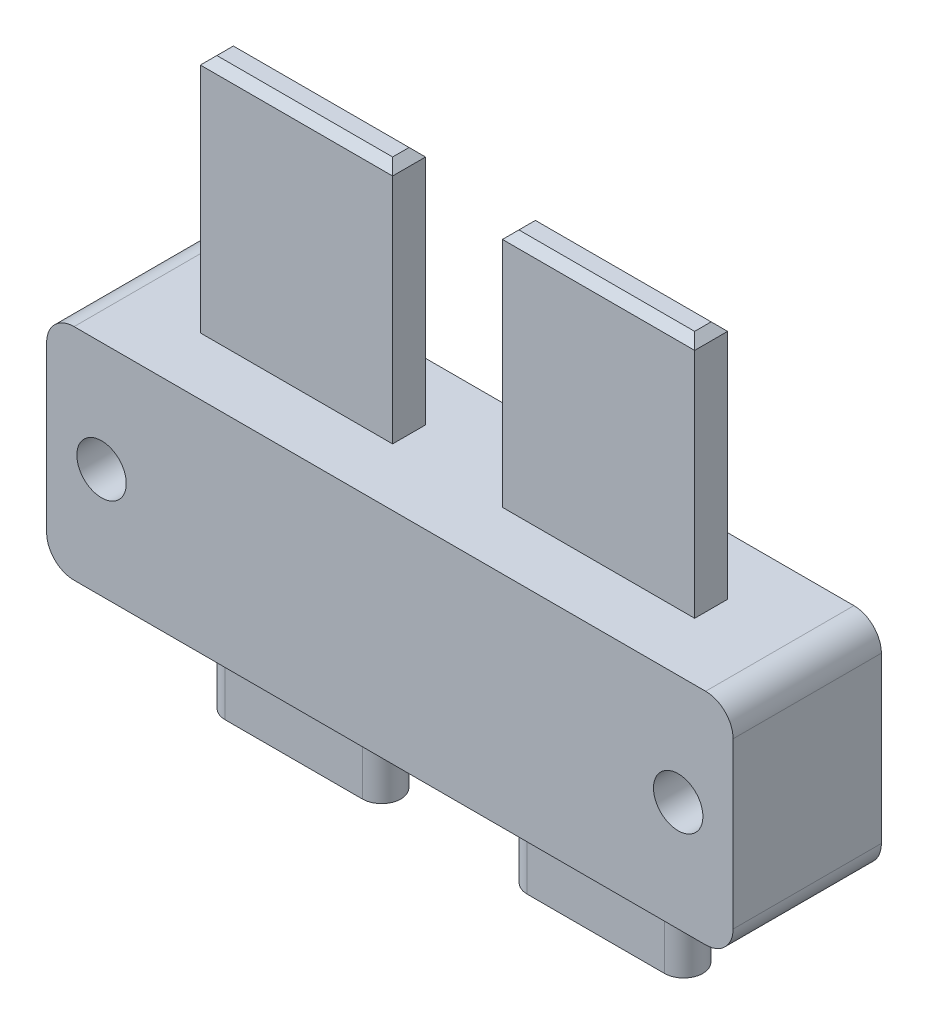
SolidWorks part; units mm, degrees
ref_plane "前视基准面" through (0, 0, 0) normal (0, 0, 1) x (1, 0, 0)
ref_plane "上视基准面" through (0, 0, 0) normal (0, 1, 0) x (1, 0, 0)
ref_plane "右视基准面" through (0, 0, 0) normal (1, 0, 0) x (0, 0, -1)
other "Configuration Table"
sketch "草图1" plane through (0, 0, 0) normal (0, 0, 1) x (1, 0, 0)
  line L0 (0, 0) -> (24.1432, 0) construction
  line L1 (-12.5, 4) -> (12.5, 4)
  line L2 (-12.5, 4) -> (-12.5, -4)
  line L3 (-12.5, -4) -> (12.5, -4)
  line L4 (12.5, 4) -> (12.5, -4)
  line L5 (-12.5, 4) -> (12.5, -4) construction
  line L6 (-12.5, -4) -> (12.5, 4) construction
  line L7 (0, 0) -> (0, 18.2924) construction
  circle A0 centre (10.5, 0) radius 0.9
  circle A1 centre (-10.5, 0) radius 0.9
  point P0 (0, 0)
  dimension "D3" = 1.8
  dimension "D4" = 21
  dimension "D1" = 8
  dimension "D2" = 25
extrude "凸台-拉伸1" add sketch "草图1" along normal blind 5.4
sketch "草图2" plane through (0, -4, 0) normal (0, -1, 0) x (-1, 0, 0)
  line L0 (0, 0) -> (0, -9.3456) construction
  line L1 (0, -2.7) -> (-16.2771, -2.7) construction
  line L2 (12.5, -5.4) -> (-12.5, -5.4) construction
  line L3 (12.5, 0) -> (-12.5, 0) construction
  line L4 (-3, -2.7) -> (-8, -2.7) construction
  line L5 (-3, -3.4) -> (-8, -3.4)
  line L6 (-3, -2) -> (-8, -2)
  line L7 (3, -2.7) -> (8, -2.7) construction
  line L8 (3, -3.4) -> (8, -3.4)
  line L9 (3, -2) -> (8, -2)
  arc A0 (-3, -3.4) -> (-3, -2) centre (-3, -2.7) ccw
  arc A1 (-8, -2) -> (-8, -3.4) centre (-8, -2.7) ccw
  arc A2 (3, -3.4) -> (3, -2) centre (3, -2.7) cw
  arc A3 (8, -2) -> (8, -3.4) centre (8, -2.7) cw
  point P11 (-5.5, -2.7)
  point P18 (5.5, -2.7)
  dimension "D3" = 11
  dimension "D1" = 5
  dimension "D2" = 1.4
extrude "凸台-拉伸2" add sketch "草图2" along normal blind 3.65
sketch "草图3" plane through (0, 4, 0) normal (0, 1, 0) x (1, 0, 0)
  line L0 (0, 0) -> (0, -7.6392) construction
  line L1 (0, -2.7) -> (15.3733, -2.7) construction
  line L2 (12.5, 0) -> (-12.5, 0) construction
  line L3 (12.5, -5.4) -> (-12.5, -5.4) construction
  line L4 (-2, -3.3) -> (-9, -2.1) construction
  line L5 (2, -2.1) -> (9, -2.1)
  line L6 (2, -2.1) -> (2, -3.3)
  line L7 (2, -3.3) -> (9, -3.3)
  line L8 (9, -2.1) -> (9, -3.3)
  line L9 (2, -2.1) -> (9, -3.3) construction
  line L10 (2, -3.3) -> (9, -2.1) construction
  line L11 (-2, -2.1) -> (-9, -3.3) construction
  line L12 (-9, -2.1) -> (-9, -3.3)
  line L13 (-2, -3.3) -> (-9, -3.3)
  line L14 (-2, -2.1) -> (-2, -3.3)
  line L15 (-2, -2.1) -> (-9, -2.1)
  point P9 (5.5, -2.7)
  point P18 (-5.5, -2.7)
  dimension "D1" = 11
  dimension "D2" = 7
  dimension "D3" = 1.2
extrude "凸台-拉伸3" add sketch "草图3" along normal blind 8.75
chamfer "倒角1" distance 0.3 angle 45 8 edges at (-5.5, 12.75, 3.3) (-9, 12.75, 2.7) (-5.5, 12.75, 2.1) (-2, 12.75, 2.7) (5.5, 12.75, 3.3) (2, 12.75, 2.7) (5.5, 12.75, 2.1) (9, 12.75, 2.7)
fillet "圆角1" radius 1 4 edges at (12.5, -4, 2.7) (12.5, 4, 2.7) (-12.5, -4, 2.7) (-12.5, 4, 2.7)
